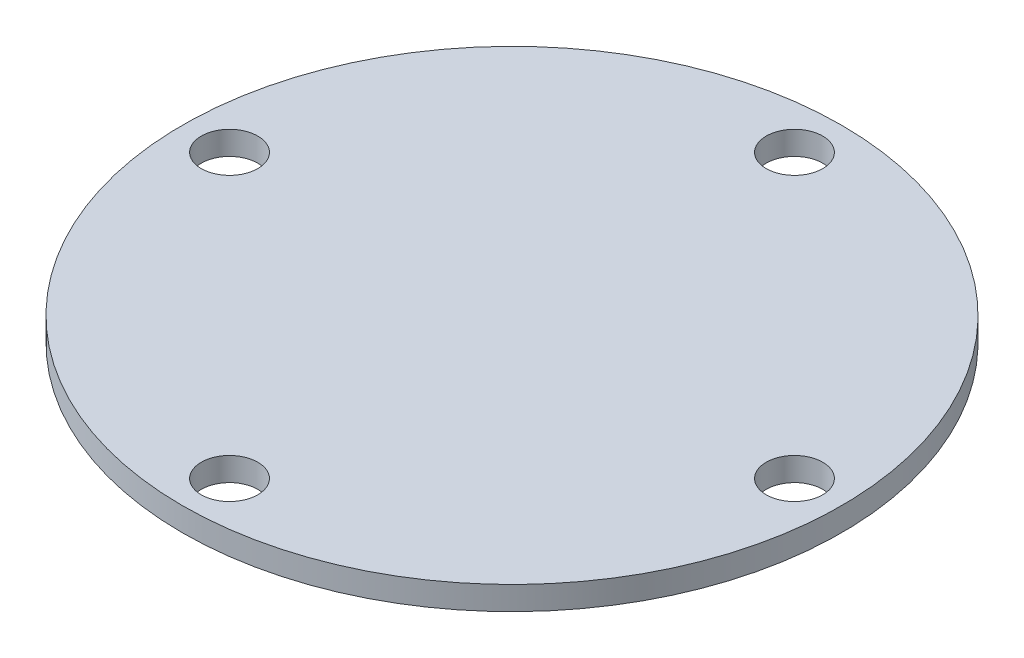
SolidWorks part; units mm, degrees
material "A3"
ref_plane "前视基准面" through (0, 0, 0) normal (0, 0, 1) x (1, 0, 0)
ref_plane "上视基准面" through (0, 0, 0) normal (0, 1, 0) x (1, 0, 0)
ref_plane "右视基准面" through (0, 0, 0) normal (1, 0, 0) x (0, 0, -1)
sketch "草图1" plane through (0, 0, 0) normal (0, 1, 0) x (1, 0, 0)
  circle A0 centre (0, 0) radius 70
  dimension "D1" = 140
extrude "凸台-拉伸1" add sketch "草图1" along normal blind 5
sketch "草图3" plane through (0, 5, 0) normal (0, 1, 0) x (1, 0, 0)
  circle A0 centre (0, 0) radius 60 construction
  circle A1 centre (0, 60) radius 6
  circle A2 centre (60, 0) radius 6
  circle A3 centre (0, -60) radius 6
  circle A4 centre (-60, 0) radius 6
  point P14 (0, 0)
  dimension "D1" = 120
  dimension "D2" = 12
  dimension "D3" = 4
extrude "切除-拉伸1" cut sketch "草图3" against normal through all
